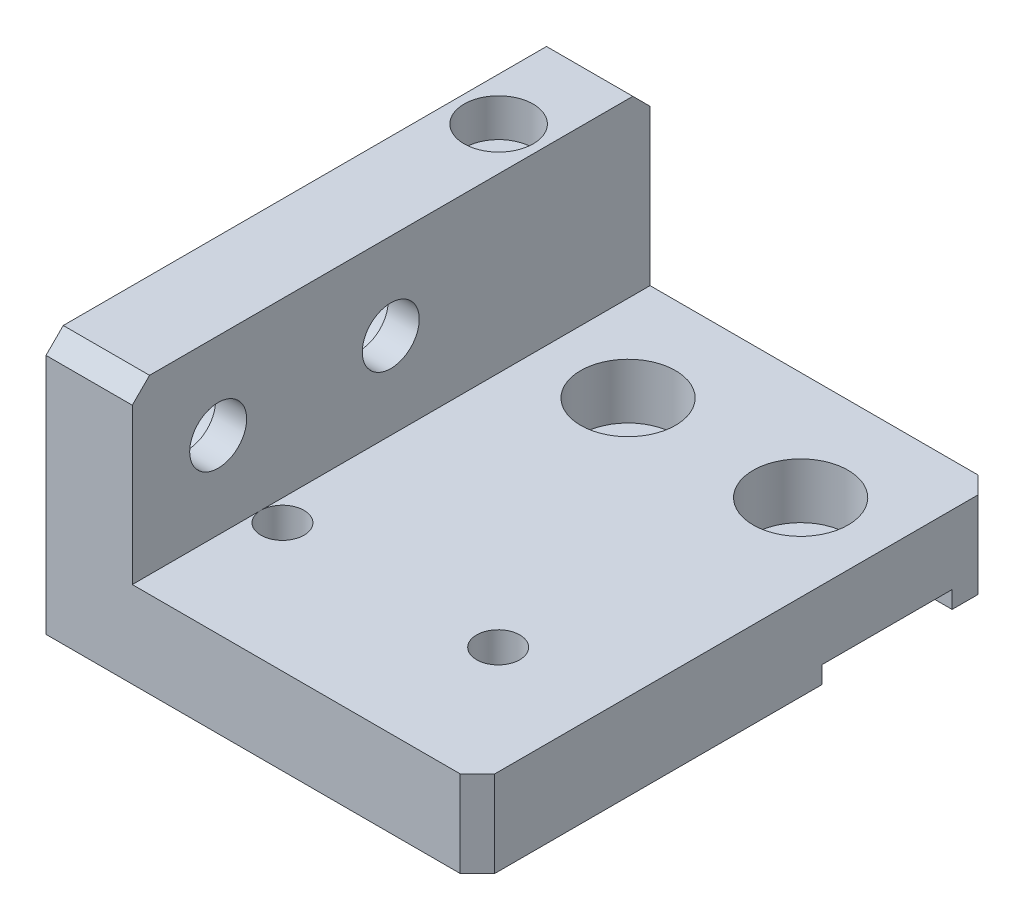
from build123d import *

# Parameters (mm, degrees)
EXTRUDE_1_DEPTH              = 60
SKETCH_3_W                   = 50
SKETCH_3_H                   = 15.1
CUT_EXTRUDE_1_DEPTH          = 2
HOLE_WIZARD_M4_1_D           = 4.5
HOLE_WIZARD_M4_1_CBORE_D     = 8
HOLE_WIZARD_M4_1_CBORE_DEPTH = 4.4
HOLE_WIZARD_M6_1_D           = 6.6
HOLE_WIZARD_M6_1_CBORE_D     = 11
HOLE_WIZARD_M6_1_CBORE_DEPTH = 6.4
HOLE_WIZARD_M6_2_D           = 6.6
HOLE_WIZARD_M6_2_CBORE_D     = 11
HOLE_WIZARD_M6_2_CBORE_DEPTH = 6.4
CHAMFER_1_SIZE               = 2
HOLE_WIZARD_M6_1_2_D         = 5
HOLE_WIZARD_M6_1_2_DEPTH     = 17
HOLE_WIZARD_M6_1_2_TIP       = 1.502151548


with BuildPart() as part:
    # 草图2 → 凸台-拉伸1 (new body)
    with BuildSketch(Plane.XY):
        Polygon((50, 0), (0, 0), (0, 30), (10, 30), (10, 10), (50, 10), align=None)
    extrude(amount=EXTRUDE_1_DEPTH)

    # 草图3 → 切除-拉伸1 (cut)
    with BuildSketch(Plane.XZ):
        with Locations((25, 12.55)):
            Rectangle(SKETCH_3_W, SKETCH_3_H)
    extrude(amount=-CUT_EXTRUDE_1_DEPTH, mode=Mode.SUBTRACT)

    # M4 六角凹头螺钉的柱形沉头孔1 (through all)
    with Locations(Plane(origin=(0, 30, 0), x_dir=(1, 0, 0), z_dir=(0, 1, 0))):
        with Locations((5, -12.55)):
            CounterBoreHole(HOLE_WIZARD_M4_1_D / 2, HOLE_WIZARD_M4_1_CBORE_D / 2, HOLE_WIZARD_M4_1_CBORE_DEPTH)

    # Hole Wizard M6 _1 (through all)
    with Locations(Plane(origin=(0, 10, 0), x_dir=(1, 0, 0), z_dir=(0, 1, 0))):
        with Locations((20, -12.55), (40, -12.55)):
            CounterBoreHole(HOLE_WIZARD_M6_1_D / 2, HOLE_WIZARD_M6_1_CBORE_D / 2, HOLE_WIZARD_M6_1_CBORE_DEPTH)

    # M6 六角凹头螺钉的柱形沉头孔2 (through all)
    with Locations(Plane.ZY):
        with Locations((30.05, 20), (50.05, 20)):
            CounterBoreHole(HOLE_WIZARD_M6_2_D / 2, HOLE_WIZARD_M6_2_CBORE_D / 2, HOLE_WIZARD_M6_2_CBORE_DEPTH)

    # 倒角1
    chamfer_1_edges = [part.edges().sort_by_distance(p)[0] for p in [
        (5, 30, 60),
        (50, 5, 60),
        (5, 30, 0),
        (50, 5, 0),
    ]]
    chamfer(chamfer_1_edges, length=CHAMFER_1_SIZE)

    # Hole Wizard M6 _1 2
    with Locations(Plane(origin=(0, 0, 0), x_dir=(-1, 0, 0), z_dir=(0, -1, 0))):
        with Locations((-37.5, -45.1), (-12.5, -45.1)):
            Hole(HOLE_WIZARD_M6_1_2_D / 2, depth=HOLE_WIZARD_M6_1_2_DEPTH)
            with Locations((0, 0, -(HOLE_WIZARD_M6_1_2_DEPTH + HOLE_WIZARD_M6_1_2_TIP / 2))):  # 118° drill point
                Cone(0, HOLE_WIZARD_M6_1_2_D / 2, HOLE_WIZARD_M6_1_2_TIP, mode=Mode.SUBTRACT)


solid = part.part
